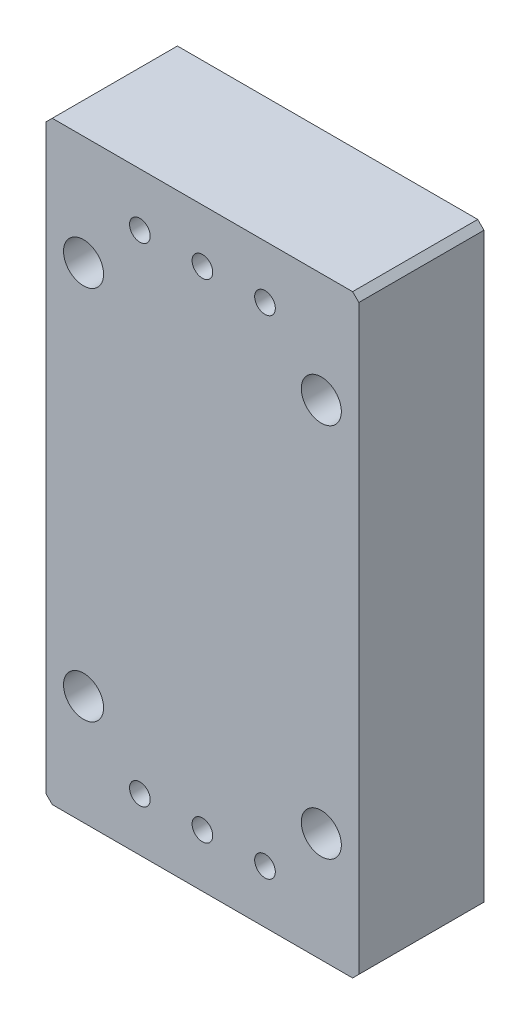
SolidWorks part; units mm, degrees
material "6061铝"
ref_plane "前视基准面" through (0, 0, 0) normal (0, 0, 1) x (1, 0, 0)
ref_plane "上视基准面" through (0, 0, 0) normal (0, 1, 0) x (1, 0, 0)
ref_plane "右视基准面" through (0, 0, 0) normal (1, 0, 0) x (0, 0, -1)
sketch "草图1" plane through (0, 0, 0) normal (0, 0, 1) x (1, 0, 0)
  line L1 (-25, 47.5) -> (25, 47.5)
  line L2 (-25, 47.5) -> (-25, -47.5)
  line L3 (-25, -47.5) -> (25, -47.5)
  line L4 (25, 47.5) -> (25, -47.5)
  line L5 (-25, 47.5) -> (25, -47.5) construction
  line L6 (-25, -47.5) -> (25, 47.5) construction
  point P0 (0, 0)
  dimension "D1" = 50
  dimension "D2" = 95
extrude "凸台-拉伸1" add sketch "草图1" along normal blind 20
hole_wizard "打孔尺寸(%根据)内六角圆柱头螺钉的类型1" positions "草图2" profile "草图3" counterbore size "M6" standard "GB" end condition through all
sketch "草图2" plane through (0, 0, 0) normal (0, 0, -1) x (-1, 0, 0)
  line L0 (0, 0) -> (0, 50.3071) construction
  line L2 (0, 0) -> (-33.4481, 0) construction
  point P0 (-19, 30)
  point P2 (-19, -30)
  point P4 (19, -30)
  point P6 (19, 30)
  point P22 (0, 0)
  point P23 (0, 0)
  dimension "D1" = 60
  dimension "D2" = 38
sketch "草图3" plane through (19, 30, 0) normal (1, 0, 0) x (0, 1, 0)
  line L0 (0, 0) -> (0, 20)
  line L1 (0, 20) -> (3.2, 20)
  line L3 (3.2, 20) -> (3.2, 7)
  line L4 (3.2, 7) -> (5.5, 7)
  line L5 (5.5, 7) -> (5.5, 0)
  line L7 (5.5, 0) -> (0, 0)
  line L11 (0, -6.35) -> (0, 107.95) construction
  dimension "通孔孔直径" = 6.4
  dimension "通孔孔深度" = 20
  dimension "柱形沉头孔直径" = 11
  dimension "柱形沉头孔深度" = 7
hole_wizard "M4 螺纹孔1" positions "草图4" profile "草图6" tap size "M4" standard "GB" end condition through all
sketch "草图4" plane through (0, 0, 0) normal (0, 0, -1) x (-1, 0, 0)
  line L1 (0, 0) -> (44.8133, 0) construction
  line L2 (0, 0) -> (0, 2.9707) construction
  point P13 (10, 39)
  point P22 (10, -39)
  point P23 (-10, -39)
  point P24 (-10, 39)
  point P25 (0, 39)
  point P27 (0, -39)
  dimension "D1" = 20
  dimension "D2" = 78
sketch "草图6" plane through (0, -39, 0) normal (1, 0, 0) x (0, 1, 0)
  line L0 (0, 0) -> (0, 20)
  line L1 (0, 20) -> (1.65, 20)
  line L2 (1.65, 20) -> (1.65, 0.375)
  line L3 (1.65, 0.375) -> (2.025, 0)
  line L5 (2.025, 0) -> (0, 0)
  line L6 (-1.65, 0.375) -> (-2.025, 0) construction
  line L11 (0, -6.35) -> (0, 107.95) construction
  dimension "通孔螺纹孔钻头直径" = 3.3
  dimension "通孔螺纹孔钻头深度" = 20
  dimension "近端锥形沉头孔直径" = 4.05
  dimension "近端锥形沉头孔角度" = 90
cosmetic thread "孔螺蚊线1" parameters "D2"=4
cosmetic thread "孔螺蚊线2" parameters "D2"=4
cosmetic thread "孔螺蚊线3" parameters "D2"=4
cosmetic thread "孔螺蚊线4" parameters "D2"=4
cosmetic thread "孔螺蚊线5" parameters "D2"=4
cosmetic thread "孔螺蚊线6" parameters "D2"=4
chamfer "倒角1" distance 1 angle 45 4 edges at (25, -47.5, 10) (-25, -47.5, 10) (-25, 47.5, 10) (25, 47.5, 10)
